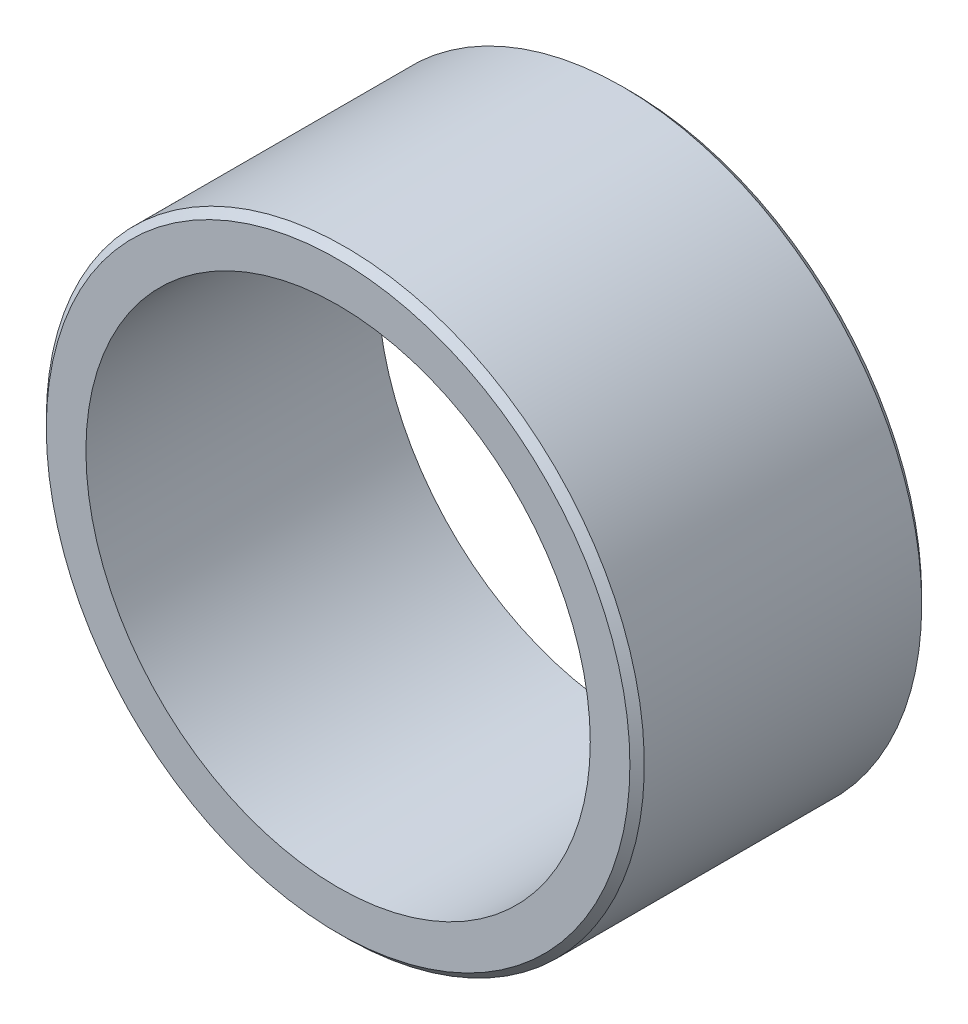
from build123d import *

# Parameters (mm, degrees)
SKETCH1_R      = 41.5
SKETCH1_R_2    = 35
EXTRUDE1_DEPTH = 40.5
CHAMFER1_SIZE  = 1


with BuildPart() as part:
    # Sketch1 → Extrude1 (new body)
    with BuildSketch(Plane.XY):
        Circle(SKETCH1_R)
        Circle(SKETCH1_R_2, mode=Mode.SUBTRACT)
    extrude(amount=EXTRUDE1_DEPTH)

    # Chamfer1
    chamfer1_edges = [part.edges().sort_by_distance(p)[0] for p in [
        (-41.5, 0, 0),
        (-41.5, 0, 40.5),
    ]]
    chamfer(chamfer1_edges, length=CHAMFER1_SIZE)


solid = part.part
